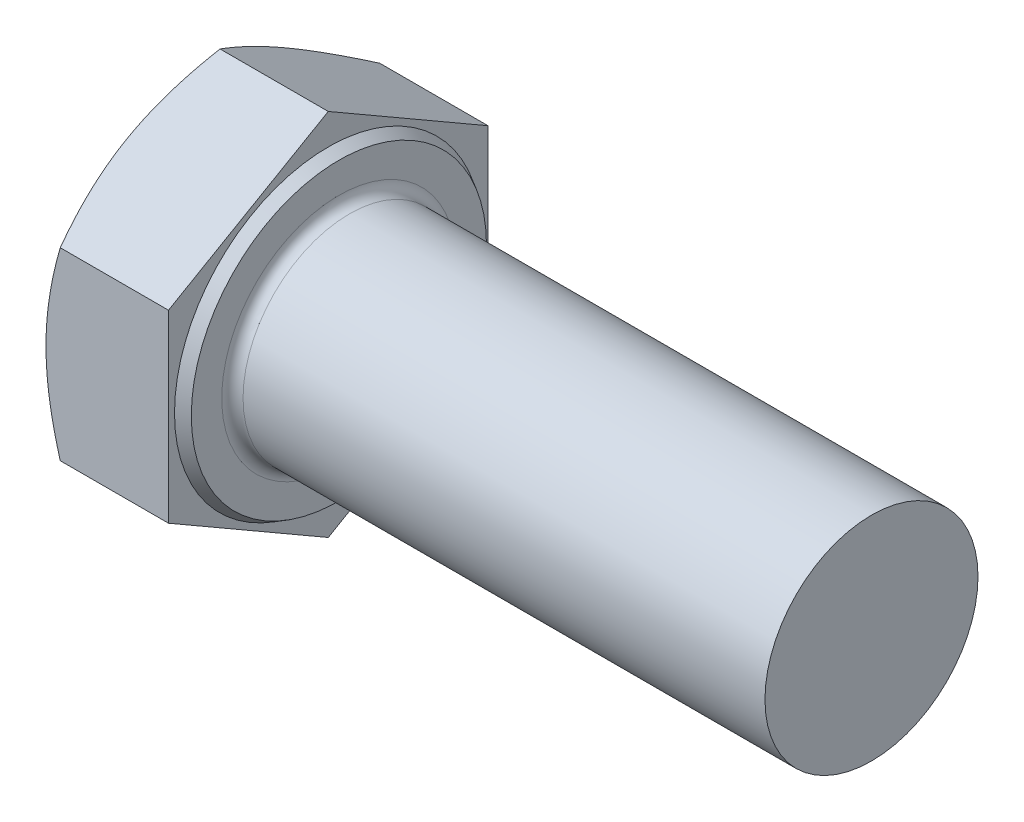
from build123d import *

# Parameters (mm, degrees)
EXTRUDE_387_DEPTH = 7.5
FILLET_1280_R     = 0.6


with BuildPart() as part:
    # 草图1 → Extrude 387 (new body)
    with BuildSketch(Plane(origin=(0, 0, 0), x_dir=(0, 0, -1), z_dir=(1, 0, 0))):
        Polygon((9, 5.196152423), (9, -5.196152423), (0, -10.392304845), (-9, -5.196152423), (-9, 5.196152423), (0, 10.392304845), align=None)
    extrude(amount=EXTRUDE_387_DEPTH)

    # 草图2 → 凸台-旋转1 (revolve)
    with BuildSketch(Plane.XY, mode=Mode.PRIVATE) as revolve_1_sk:
        Polygon((0, 0), (37.5, 0), (37.5, 4.4845), (37.5, 6), (7.5, 6), (0, 6), align=None)
    revolve(revolve_1_sk.sketch.rotate(Axis((0, 0, 0), (1, 0, 0)), 90), axis=Axis((0, 0, 0), (1, 0, 0)))

    # 草图3 → 切除-旋转1 (revolve, cut)
    with BuildSketch(Plane.XY):
        Polygon((0, 9), (3.690598923, 15.392304845), (3.690598923, 20.392304845), (-10, 20.392304845), (-10, 9), align=None)
    revolve(axis=Axis((0, 0, 0), (1, 0, 0)), mode=Mode.SUBTRACT)

    # 草图4 → 切除-旋转3 (revolve, cut)
    with BuildSketch(Plane.XY, mode=Mode.PRIVATE) as cut_revolve_3_sk:
        Polygon((7.5, 8.315), (6.9, 8.661410162), (6.9, 10.392304845), (7.5, 10.392304845), align=None)
    revolve(cut_revolve_3_sk.sketch.rotate(Axis((0, 0, 0), (1, 0, 0)), 90), axis=Axis((0, 0, 0), (1, 0, 0)), mode=Mode.SUBTRACT)

    # Fillet 1280
    fillet_1280_edges = [part.edges().sort_by_distance(p)[0] for p in [
        (7.5, 0, -6),
    ]]
    fillet(fillet_1280_edges, radius=FILLET_1280_R)


solid = part.part
